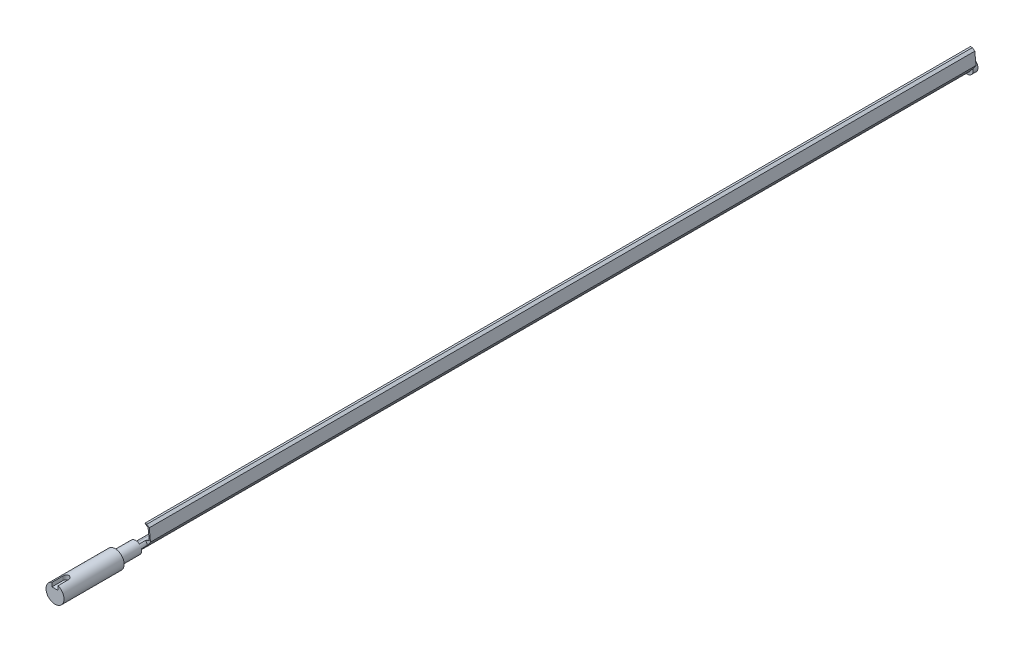
from build123d import *

# Parameters (mm, degrees)
SKETCH1_R           = 100
BOSS_EXTRUDE1_DEPTH = 340
BOSS_EXTRUDE2_DEPTH = 13824
BOSS_EXTRUDE3_START = 80
SKETCH3_R           = 100
BOSS_EXTRUDE3_DEPTH = 80
CUT_EXTRUDE1_START  = -100
CUT_EXTRUDE1_DEPTH  = 100
SKETCH6_R           = 150
BOSS_EXTRUDE5_DEPTH = 1000
CUT_EXTRUDE2_DEPTH  = 326
BOSS_EXTRUDE6_DEPTH = 75


with BuildPart() as part:
    # Sketch1 → Boss-Extrude1 (new body)
    with BuildSketch(Plane.XY):
        Circle(SKETCH1_R)
    extrude(amount=BOSS_EXTRUDE1_DEPTH)

    # Sketch2 → Boss-Extrude2 (add)
    with BuildSketch(Plane(origin=(0, 0, 0), x_dir=(-1, 0, 0), z_dir=(0, 0, -1))):
        with BuildLine():
            Line((-96.233395069, 27.187012957), (-146.428749083, 97.201990132))
            Line((-146.428749083, 97.201990132), (-127.238656611, 294.943377783))
            Line((-127.238656611, 294.943377783), (-85.855376139, 324.612007229))
            Line((-85.855376139, 324.612007229), (-53.815694107, 324.612007229))
            Line((-53.815694107, 324.612007229), (-69.835535123, 313.127013254))
            Line((-69.835535123, 313.127013254), (-106.547016375, 286.807704556))
            Line((-106.547016375, 286.807704556), (-127.238656611, 110.959810588))
            Line((-127.238656611, 110.959810588), (-61.825614615, 78.597667761))
            Line((-61.825614615, 78.597667761), (0, 58.675035722))
            ThreePointArc((0, 58.675035722), (51.995426196, -27.188885075), (-48.18736452, -33.477421012))
            Line((-48.18736452, -33.477421012), (-96.233395069, 27.187012957))
        make_face()
    extrude(amount=BOSS_EXTRUDE2_DEPTH)

    # Sketch3 → Boss-Extrude3 (add)
    with BuildSketch(Plane(origin=(0, 0, -13824), x_dir=(-1, 0, 0), z_dir=(0, 0, -1)).offset(BOSS_EXTRUDE3_START)):
        with Locations(Location((0, 0, 0), (0, 0, 128.188900559))):
            Circle(SKETCH3_R)
    extrude(amount=-BOSS_EXTRUDE3_DEPTH)

    # Sketch4 → Cut-Extrude1 (cut)
    with BuildSketch(Plane.XY.offset(CUT_EXTRUDE1_START)):
        with BuildLine():
            Line((96.233395069, 27.187012957), (146.428749083, 97.201990132))
            Line((146.428749083, 97.201990132), (127.238656611, 294.943377783))
            Line((127.238656611, 294.943377783), (85.855376139, 324.612007229))
            Line((85.855376139, 324.612007229), (53.815694107, 324.612007229))
            Line((53.815694107, 324.612007229), (106.547016375, 286.807704556))
            Line((106.547016375, 286.807704556), (127.238656611, 110.959810588))
            Line((127.238656611, 110.959810588), (61.825614615, 78.597667761))
            ThreePointArc((61.825614615, 78.597667761), (83.104912565, 55.619902082), (96.233395069, 27.187012957))
        make_face()
    extrude(amount=CUT_EXTRUDE1_DEPTH, mode=Mode.SUBTRACT)

    # Sketch6 → Boss-Extrude5 (add)
    with BuildSketch(Plane.XY.offset(340)):
        Circle(SKETCH6_R)
    extrude(amount=BOSS_EXTRUDE5_DEPTH)

    # Sketch7 → Cut-Extrude2 (cut)
    with BuildSketch(Plane(origin=(0, 0, 0), x_dir=(1, 0, 0), z_dir=(0, 1, 0))):
        with BuildLine():
            Line((50, -1160), (50, -1460))
            ThreePointArc((50, -1460), (0, -1510), (-50, -1460))
            Line((-50, -1460), (-50, -1160))
            ThreePointArc((-50, -1160), (0, -1110), (50, -1160))
        make_face()
    extrude(amount=CUT_EXTRUDE2_DEPTH, mode=Mode.SUBTRACT)

    # Sketch8 → Boss-Extrude6 (add)
    with BuildSketch(Plane(origin=(0, 0, 0), x_dir=(1, 0, 0), z_dir=(0, 1, 0))):
        with BuildLine():
            Line((-50, -1160), (-50, -1340))
            Line((-50, -1340), (50, -1340))
            Line((50, -1340), (50, -1160))
            ThreePointArc((50, -1160), (0, -1110), (-50, -1160))
        make_face()
    extrude(amount=BOSS_EXTRUDE6_DEPTH)


solid = part.part
